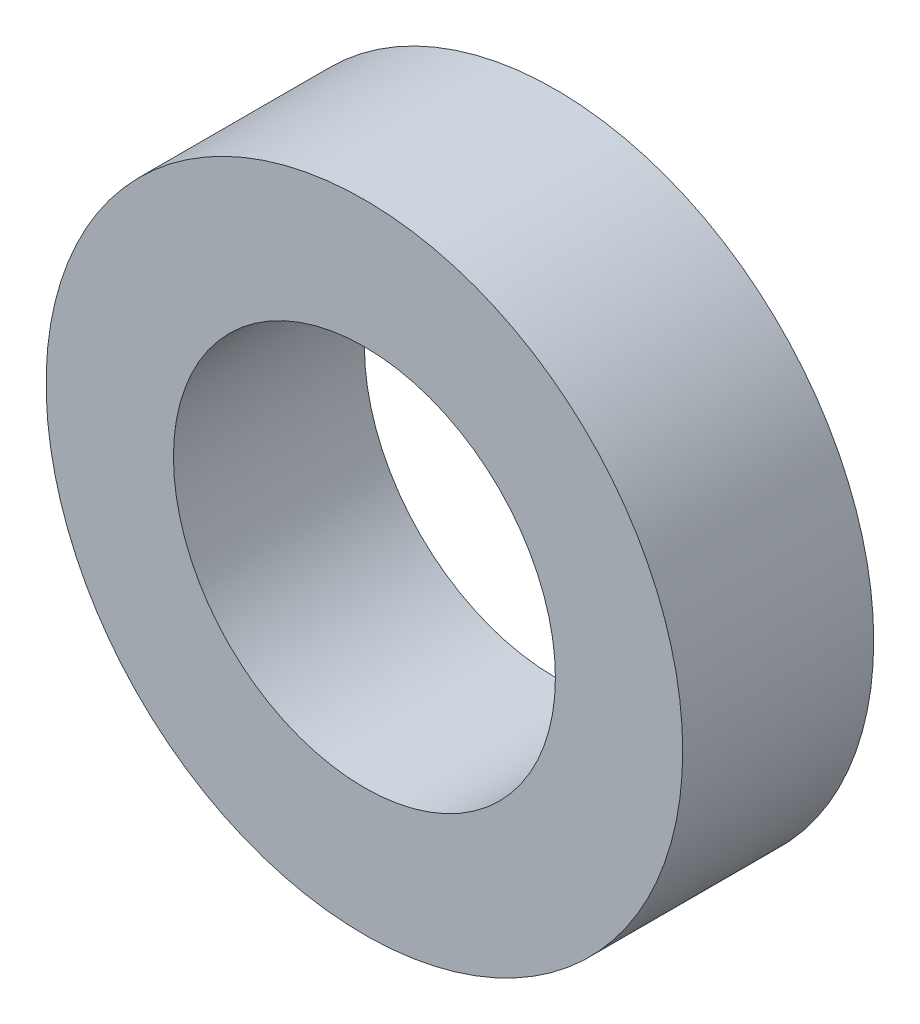
SolidWorks part; units mm, degrees
ref_plane "Front Plane" through (0, 0, 0) normal (0, 0, 1) x (1, 0, 0)
ref_plane "Top Plane" through (0, 0, 0) normal (0, 1, 0) x (1, 0, 0)
ref_plane "Right Plane" through (0, 0, 0) normal (1, 0, 0) x (0, 0, -1)
sketch "Sketch1" plane through (0, 0, 0) normal (0, 0, 1) x (1, 0, 0)
  circle A0 centre (0, 0) radius 10
  circle A1 centre (0, 0) radius 6
  dimension "D1" = 20
  dimension "D2" = 12
extrude "Boss-Extrude1" add sketch "Sketch1" along normal mid plane 6
